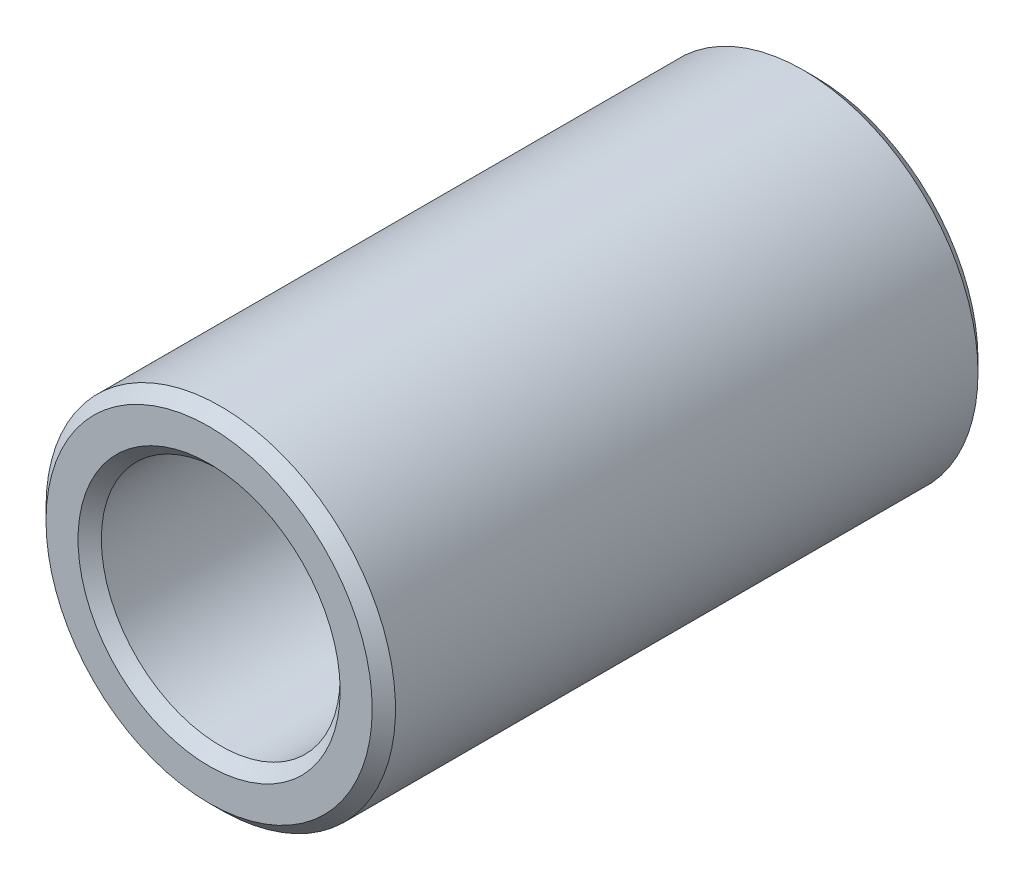
from build123d import *

# Parameters (mm, degrees)
SKETCH_1_R      = 15
SKETCH_1_R_2    = 10.25
EXTRUDE_1_DEPTH = 26
CHAMFER_1_SIZE  = 1


with BuildPart() as part:
    # 草图1 → 凸台-拉伸1 (new, symmetric)
    with BuildSketch(Plane.XY):
        with Locations(Location((0, 0, 0), (0, 0, 180))):
            Circle(SKETCH_1_R)
        with Locations(Location((0, 0, 0), (0, 0, 180))):
            Circle(SKETCH_1_R_2, mode=Mode.SUBTRACT)
    extrude(amount=EXTRUDE_1_DEPTH, both=True)

    # 倒角1
    chamfer_1_edges = [part.edges().sort_by_distance(p)[0] for p in [
        (15, 0, -26),
        (15, 0, 26),
        (10.25, 0, -26),
        (10.25, 0, 26),
    ]]
    chamfer(chamfer_1_edges, length=CHAMFER_1_SIZE)


solid = part.part
